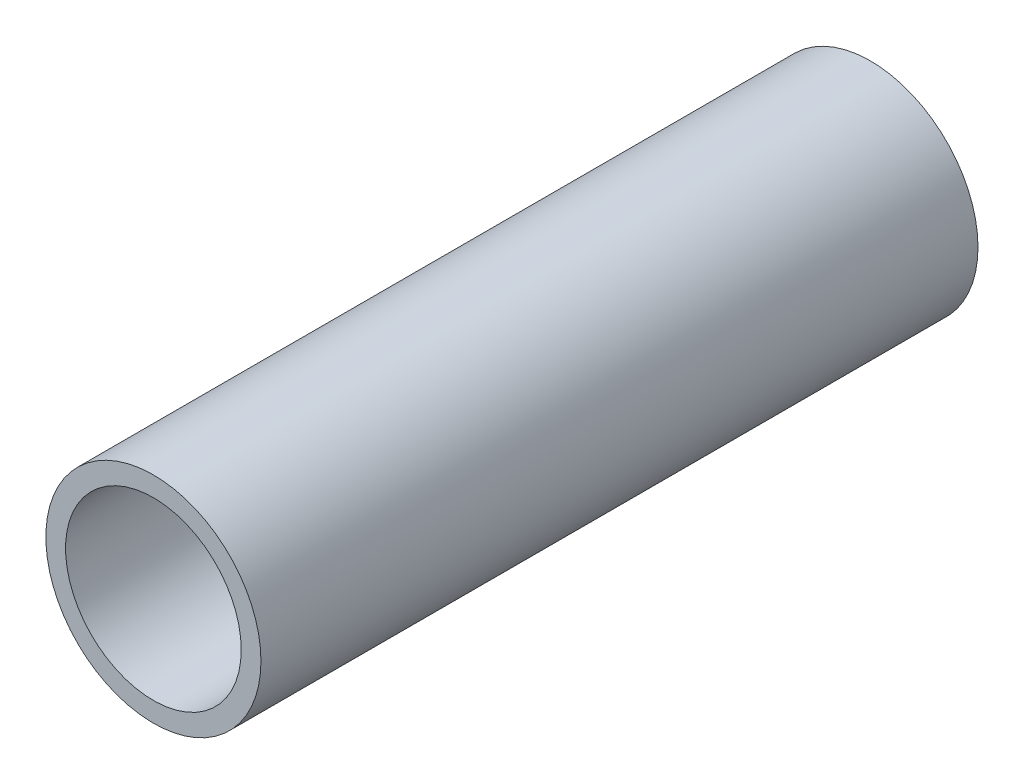
SolidWorks part; units mm, degrees
ref_plane "前视基准面" through (0, 0, 0) normal (0, 0, 1) x (1, 0, 0)
ref_plane "上视基准面" through (0, 0, 0) normal (0, 1, 0) x (1, 0, 0)
ref_plane "右视基准面" through (0, 0, 0) normal (1, 0, 0) x (0, 0, -1)
sketch "草图1" plane through (0, 0, 0) normal (0, 0, 1) x (1, 0, 0)
  circle A0 centre (0, 0) radius 2.45
  circle A1 centre (0, 0) radius 3
extrude "凸台-拉伸1" add sketch "草图1" against normal up to surface (20 mm away)
